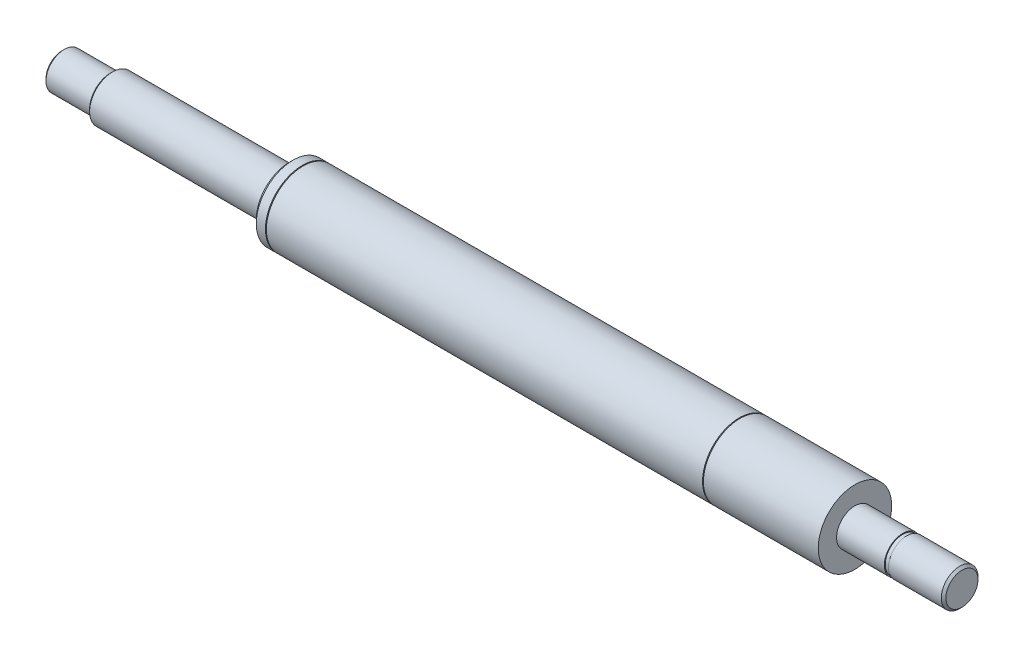
SolidWorks part; units mm, degrees
ref_plane "Front" through (0, 0, 0) normal (0, 0, 1) x (1, 0, 0)
ref_plane "Top" through (0, 0, 0) normal (0, 1, 0) x (1, 0, 0)
ref_plane "Right" through (0, 0, 0) normal (1, 0, 0) x (0, 0, -1)
sketch "Sketch1" plane through (0, 0, 0) normal (0, 1, 0) x (1, 0, 0)
  line L0 (-12.2567, 0) -> (202.5999, 0) construction
  line L1 (0, 0) -> (0, -4)
  line L2 (0, -4) -> (10.5, -4)
  line L3 (10.5, -4) -> (10.5, -5)
  line L4 (10.5, -5) -> (49.5, -5)
  line L5 (49.5, -5) -> (49.5, -8)
  line L6 (49.5, -8) -> (172.7, -8)
  line L7 (172.7, -8) -> (172.7, -4)
  line L8 (172.7, -4) -> (196, -4)
  line L9 (196, -4) -> (196, 0)
  line L10 (196, 0) -> (0, 0)
  dimension "D1" = 23.3
  dimension "D2" = 123.2
  dimension "D3" = 39
  dimension "D4" = 10.5
  dimension "D5" = 8
  dimension "D6" = 10
  dimension "D7" = 16
  dimension "D8" = 8
revolve "Revolve1" add sketch "Sketch1" angle 360 mid plane about L0
sketch "Sketch2" plane through (0, 0, 0) normal (0, 1, 0) x (1, 0, 0)
  line L0 (-6.3552, 0) -> (198.6277, 0) construction
  line L1 (49.5, -8) -> (172.7, -8) construction
  line L2 (52.3, -8) -> (52.5, -8)
  line L3 (52.3, -8) -> (52.3, -6.4)
  line L4 (52.3, -6.4) -> (52.5, -6.4)
  line L5 (52.5, -8) -> (52.5, -6.4)
  line L6 (49.5, -8) -> (172.7, -8) construction
  line L7 (147.5, -8) -> (147.7, -8)
  line L8 (147.5, -8) -> (147.5, -6.4)
  line L9 (147.5, -6.4) -> (147.7, -6.4)
  line L10 (147.7, -8) -> (147.7, -6.4)
  line L11 (172.7, -4) -> (196, -4) construction
  line L12 (183.1, -4) -> (184, -4)
  line L13 (183.1, -4) -> (183.1, -3.8)
  line L14 (183.1, -3.8) -> (184, -3.8)
  line L15 (184, -4) -> (184, -3.8)
  dimension "D1" = 52.5
  dimension "D2" = 0.2
  dimension "D3" = 95
  dimension "D4" = 12.8
  dimension "D5" = 35.6
  dimension "D6" = 0.9
  dimension "D7" = 7.6
revolve "Cut-Revolve1" cut sketch "Sketch2" angle 360 mid plane about L0
chamfer "Chamfer1" distance 0.5 angle 45 3 edges at (10.5, 0, 5) (0, 0, 4) (196, 0, 4)
chamfer "Chamfer2" distance 0.8 angle 45 1 edges at (49.5, 0, 8)
